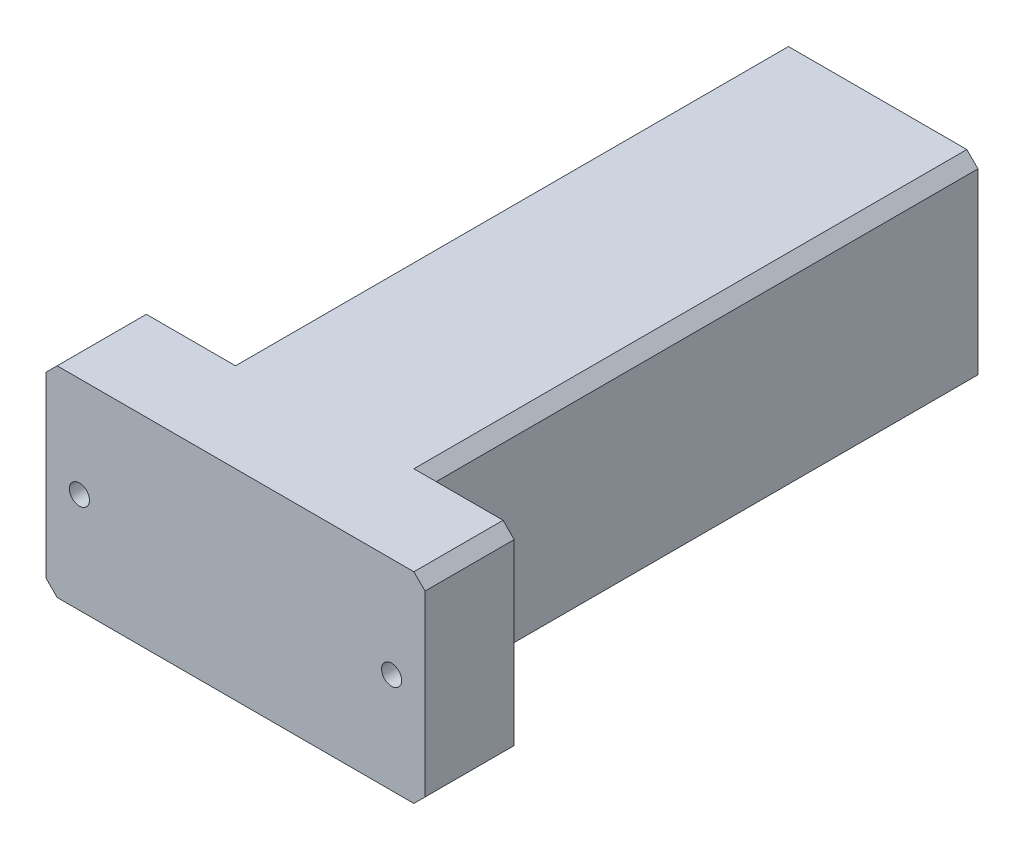
SolidWorks part; units mm, degrees
material "S45C"
ref_plane "Front Plane" through (0, 0, 0) normal (0, 0, 1) x (1, 0, 0)
ref_plane "Top Plane" through (0, 0, 0) normal (0, 1, 0) x (1, 0, 0)
ref_plane "Right Plane" through (0, 0, 0) normal (1, 0, 0) x (0, 0, -1)
sketch "Sketch1" plane through (0, 0, 0) normal (0, 0, 1) x (1, 0, 0)
  line L1 (-45, 45) -> (45, 45)
  line L2 (-45, 45) -> (-45, -45)
  line L3 (-45, -45) -> (45, -45)
  line L4 (45, 45) -> (45, -45)
  line L5 (-45, 45) -> (45, -45) construction
  line L6 (-45, -45) -> (45, 45) construction
  point P0 (0, 0)
  dimension "D1" = 90
  dimension "D2" = 90
extrude "Boss-Extrude1" add sketch "Sketch1" along normal blind 288
sketch "Sketch2" plane through (0, 0, 288) normal (0, 0, 1) x (1, 0, 0)
  line L0 (45, 45) -> (-45, 45) construction
  line L1 (85, -45) -> (-85, -45)
  line L2 (85, -45) -> (85, 45)
  line L3 (85, 45) -> (-85, 45)
  line L4 (-85, -45) -> (-85, 45)
  line L5 (85, -45) -> (-85, 45) construction
  line L6 (85, 45) -> (-85, -45) construction
  line L7 (-45, 45) -> (-45, -45) construction
  point P0 (0, 0)
  dimension "D1" = 40
extrude "Boss-Extrude2" add sketch "Sketch2" against normal blind 40
chamfer "Chamfer1" distance 5 angle 45 8 edges at (-45, -45, 124) (-45, 45, 124) (45, -45, 124) (45, 45, 124) (85, 45, 268) (85, -45, 268) (-85, 45, 268) (-85, -45, 268)
hole_wizard "M8 Clearance Hole1" positions "Sketch5" profile "Sketch4" hole size "M8" standard "GB" end condition through all
sketch "Sketch5" plane through (0, 0, 248) normal (0, 0, -1) x (-1, 0, 0)
  line L0 (0, 500) -> (0, -500) construction
  line L1 (-500, 0) -> (500, 0) construction
  point P5 (70, 0)
  point P7 (-70, 0)
  dimension "D1" = 140
sketch "Sketch4" plane through (70, 0, 248) normal (1, 0, 0) x (0, 1, 0)
  line L0 (0, 0) -> (0, 40)
  line L1 (0, 40) -> (4.5, 40)
  line L2 (4.5, 40) -> (4.5, 0)
  line L5 (4.5, 0) -> (0, 0)
  line L11 (0, -6.35) -> (0, 107.95) construction
  dimension "通孔孔直径" = 9
  dimension "通孔孔深度" = 40
